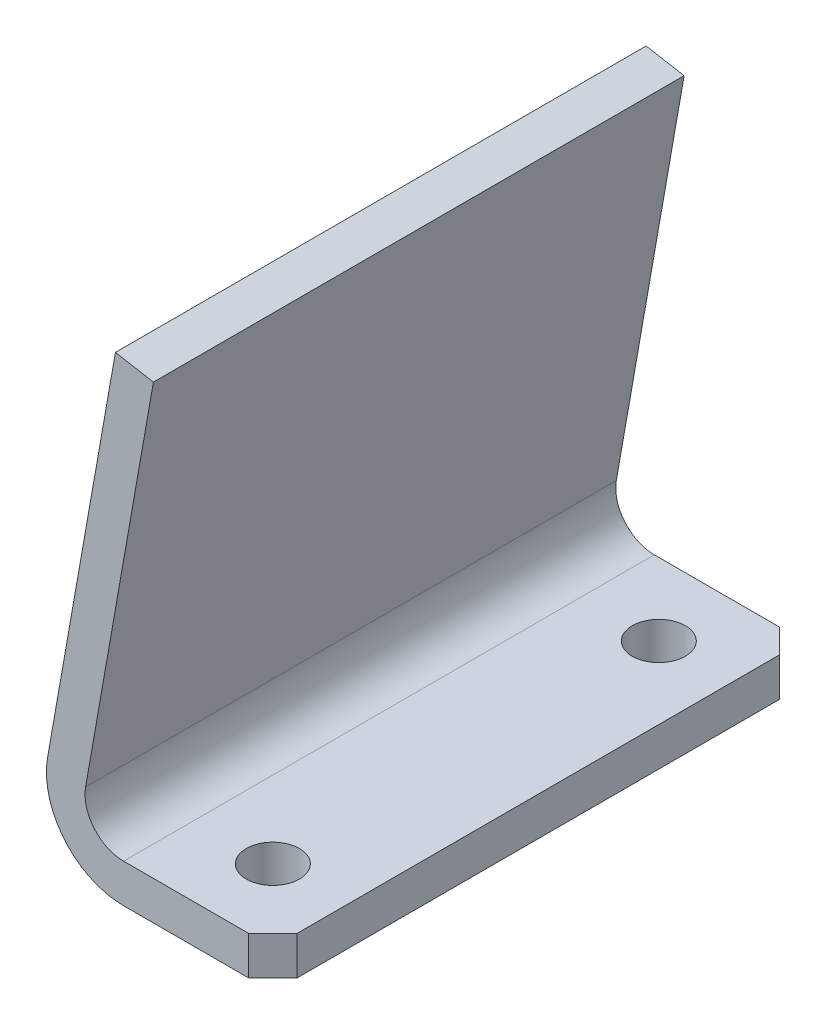
from build123d import *

# Parameters (mm, degrees)
EXTRUDE_1_DEPTH         = 110
CUT_EXTRUDE_1_DEPTH     = 156.879643007
HOLE_WIZARD_11_0_11_1_D = 11
CHAMFER_1_SIZE          = 5
FILLET_1_R              = 8
FILLET_2_R              = 16


with BuildPart() as part:
    # 草图1 → 凸台-拉伸1 (new body)
    with BuildSketch(Plane.XY.offset(110)):
        Polygon((50, 0), (50, 92.726312153), (17.364817767, 98.480775301), (0, 0), align=None)
    extrude(amount=-EXTRUDE_1_DEPTH)

    # 草图2 → 切除-拉伸1 (cut, through all)
    with BuildSketch(Plane(origin=(0, 0, 0), x_dir=(-1, 0, 0), z_dir=(0, 0, -1))):
        Polygon((-9.534028741, 8), (-25.243279791, 97.09158988), (-50, 92.726312153), (-50, 8), align=None)
    extrude(amount=-CUT_EXTRUDE_1_DEPTH, mode=Mode.SUBTRACT)

    # Ø11.0 (11) 直径孔1 (through all)
    with Locations(Plane(origin=(0, 8, 0), x_dir=(1, 0, 0), z_dir=(0, 1, 0))):
        with Locations((35, -15), (35, -95)):
            Hole(HOLE_WIZARD_11_0_11_1_D / 2)

    # 倒角1
    chamfer_1_edges = [part.edges().sort_by_distance(p)[0] for p in [
        (50, 4, 110),
        (50, 4, 0),
    ]]
    chamfer(chamfer_1_edges, length=CHAMFER_1_SIZE)

    # 圆角1
    fillet_1_edges = [part.edges().sort_by_distance(p)[0] for p in [
        (9.534028741, 8, 55),
    ]]
    fillet(fillet_1_edges, radius=FILLET_1_R)

    # 圆角2
    fillet_2_edges = [part.edges().sort_by_distance(p)[0] for p in [
        (0, 0, 55),
    ]]
    fillet(fillet_2_edges, radius=FILLET_2_R)


solid = part.part
